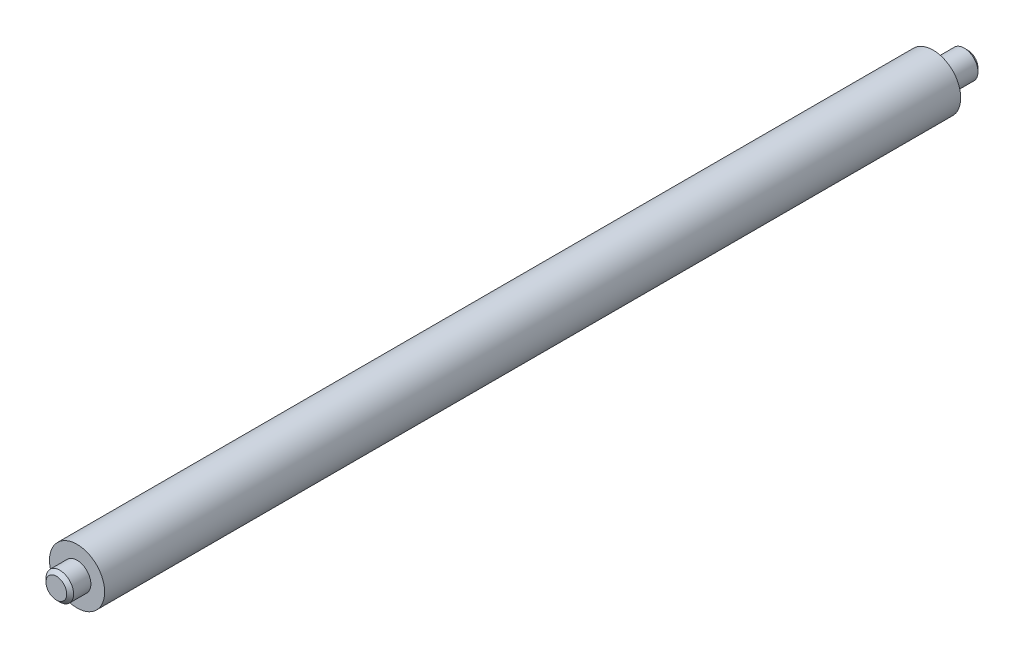
from build123d import *

# Parameters (mm, degrees)
SKETCH1_R           = 8
BOSS_EXTRUDE1_DEPTH = 248
SKETCH2_R           = 4
BOSS_EXTRUDE2_DEPTH = 10
BOSS_EXTRUDE3_START = 6
SKETCH3_R           = 4
BOSS_EXTRUDE3_DEPTH = 6
CHAMFER1_SIZE       = 1


with BuildPart() as part:
    # Sketch1 → Boss-Extrude1 (new body)
    with BuildSketch(Plane.XY):
        Circle(SKETCH1_R)
    extrude(amount=BOSS_EXTRUDE1_DEPTH)

    # Sketch2 → Boss-Extrude2 (add)
    with BuildSketch(Plane(origin=(0, 0, 0), x_dir=(-1, 0, 0), z_dir=(0, 0, -1))):
        with Locations(Location((0, 0, 0), (0, 0, 180))):
            Circle(SKETCH2_R)
    extrude(amount=BOSS_EXTRUDE2_DEPTH)

    # Sketch3 → Boss-Extrude3 (add)
    with BuildSketch(Plane.XY.offset(248).offset(BOSS_EXTRUDE3_START)):
        Circle(SKETCH3_R)
    extrude(amount=-BOSS_EXTRUDE3_DEPTH)

    # Chamfer1
    chamfer1_edges = [part.edges().sort_by_distance(p)[0] for p in [
        (-4, 0, 254),
        (-4, 0, -10),
    ]]
    chamfer(chamfer1_edges, length=CHAMFER1_SIZE)


solid = part.part
